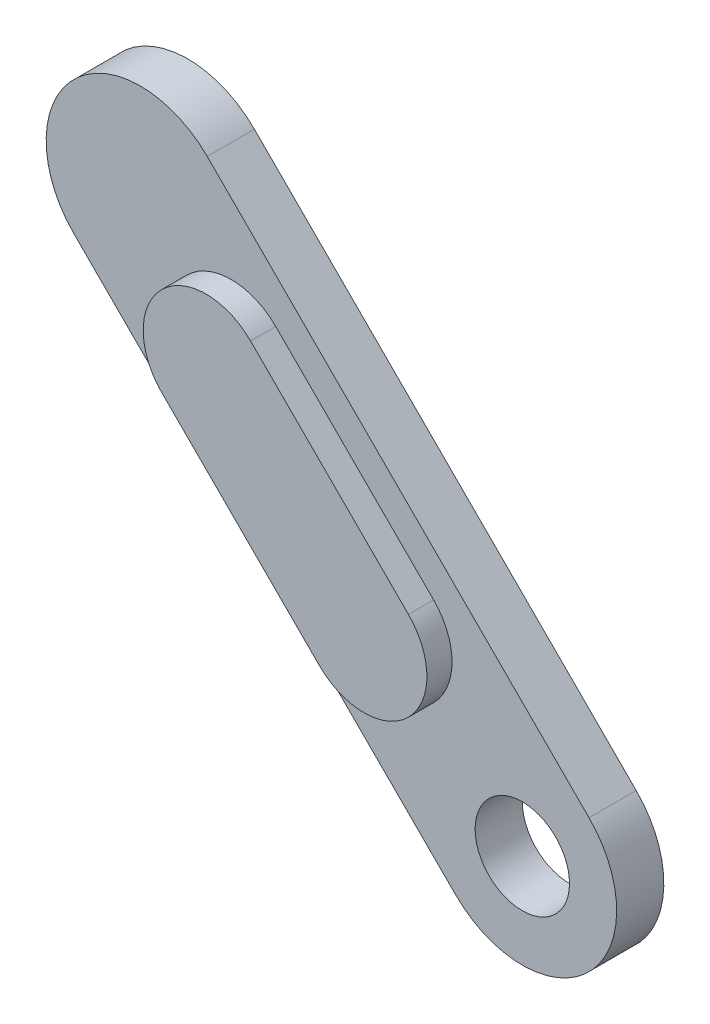
from build123d import *

# Parameters (mm, degrees)
BOSS_EXTRUDE1_DEPTH = 1.5
BOSS_EXTRUDE3_DEPTH = 0.8
SKETCH4_R           = 1.5
CUT_EXTRUDE1_DEPTH  = 0.8
CUT_EXTRUDE2_START  = -0.5
SKETCH5_R           = 1.5
CUT_EXTRUDE2_DEPTH  = 13
SKETCH6_R           = 1.5
CUT_EXTRUDE3_DEPTH  = 7


with BuildPart() as part:
    # Sketch2 → Boss-Extrude1 (new body)
    with BuildSketch(Plane.XY):
        with BuildLine():
            Line((7.699872028, 39.883123683), (-4.438596359, 52.02159207))
            ThreePointArc((-4.438596359, 52.02159207), (-8.681237046, 52.02159207), (-8.681237046, 47.778951383))
            Line((-8.681237046, 47.778951383), (3.457231341, 35.640482996))
            ThreePointArc((3.457231341, 35.640482996), (7.699872028, 35.640482996), (7.699872028, 39.883123683))
        make_face()
    extrude(amount=BOSS_EXTRUDE1_DEPTH)

    # Sketch3 → Boss-Extrude3 (add)
    with BuildSketch(Plane.XY.offset(1.5)):
        with BuildLine():
            Line((-2.260895514, 48.429677662), (2.758792127, 43.409990022))
            ThreePointArc((2.758792127, 43.409990022), (2.758792127, 40.581562897), (-0.069634998, 40.581562897))
            Line((-0.069634998, 40.581562897), (-5.089322639, 45.601250538))
            ThreePointArc((-5.089322639, 45.601250538), (-5.089322639, 48.429677662), (-2.260895514, 48.429677662))
        make_face()
    extrude(amount=BOSS_EXTRUDE3_DEPTH)

    # Sketch4 → Cut-Extrude1 (cut)
    with BuildSketch(Plane(origin=(0, 0, 0), x_dir=(-1, 0, 0), z_dir=(0, 0, -1))):
        with Locations((-5.578551684, 37.761803339)):
            Circle(SKETCH4_R)
    extrude(amount=-CUT_EXTRUDE1_DEPTH, mode=Mode.SUBTRACT)

    # Sketch5 → Cut-Extrude2 (cut)
    with BuildSketch(Plane.XY.offset(1.5).offset(CUT_EXTRUDE2_START)):
        with Locations((-6.559916703, 49.900271726)):
            Circle(SKETCH5_R)
    extrude(amount=-CUT_EXTRUDE2_DEPTH, mode=Mode.SUBTRACT)

    # Sketch6 → Cut-Extrude3 (cut)
    with BuildSketch(Plane(origin=(0, 0, 0), x_dir=(-1, 0, 0), z_dir=(0, 0, -1))):
        with Locations((-5.578551684, 37.761803339)):
            Circle(SKETCH6_R)
    extrude(amount=-CUT_EXTRUDE3_DEPTH, mode=Mode.SUBTRACT)


solid = part.part
